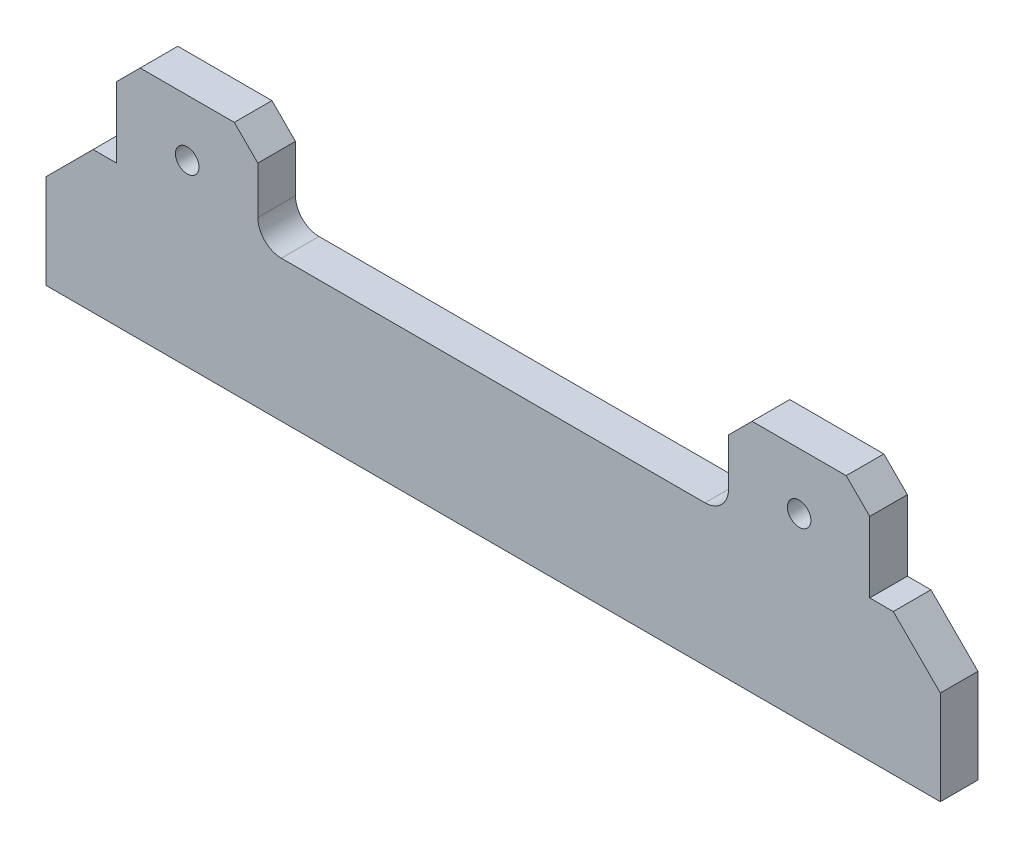
SolidWorks part; units mm, degrees
ref_plane "前视基准面" through (0, 0, 0) normal (0, 0, 1) x (1, 0, 0)
ref_plane "上视基准面" through (0, 0, 0) normal (0, 1, 0) x (1, 0, 0)
ref_plane "右视基准面" through (0, 0, 0) normal (1, 0, 0) x (0, 0, -1)
sketch "草图1" plane through (0, 0, 0) normal (0, 0, 1) x (1, 0, 0)
  line L1 (95, 25) -> (-95, 25)
  line L2 (95, 25) -> (95, -25)
  line L3 (95, -25) -> (-95, -25)
  line L4 (-95, 25) -> (-95, -25)
  line L5 (95, 25) -> (-95, -25) construction
  line L6 (95, -25) -> (-95, 25) construction
  point P0 (0, 0)
  dimension "D1" = 190
  dimension "D2" = 50
extrude "凸台-拉伸1" add sketch "草图1" along normal blind 8
sketch "草图2" plane through (0, 0, 8) normal (0, 0, 1) x (1, 0, 0)
  line L0 (-95, 25) -> (-95, -25) construction
  line L1 (-95, -5) -> (-85, 5)
  line L2 (-85, 5) -> (-80, 5)
  line L3 (-80, 5) -> (-80, 25)
  line L4 (95, 25) -> (-95, 25) construction
  line L5 (-80, 25) -> (-50, 25)
  line L6 (-50, 25) -> (-50, 5)
  line L7 (-50, 5) -> (50, 5)
  line L8 (50, 5) -> (50, 25)
  line L9 (50, 25) -> (80, 25)
  line L10 (80, 25) -> (80, 5)
  line L11 (80, 5) -> (85, 5)
  line L12 (85, 5) -> (95, -5)
  line L13 (95, -25) -> (95, 25) construction
  line L14 (-95, -5) -> (-95, 25)
  line L15 (-95, 25) -> (-3.8011, 36.2648)
  line L16 (-3.8011, 36.2648) -> (95, 25)
  line L17 (95, 25) -> (95, -5)
  dimension "D1" = 10
  dimension "D2" = 10
  dimension "D3" = 10
  dimension "D4" = 10
  dimension "D5" = 100
  dimension "D6" = 30
  dimension "D7" = 30
  dimension "D8" = 5
  dimension "D9" = 20
extrude "切除-拉伸1" cut sketch "草图2" against normal blind 8
chamfer "倒角1" distance 5 angle 45 4 edges at (80, 25, 4) (-50, 25, 4) (50, 25, 4) (-80, 25, 4)
sketch "草图3" plane through (0, 0, 8) normal (0, 0, 1) x (1, 0, 0)
  line L0 (-55, 25) -> (-75, 25) construction
  circle A0 centre (-65, 13) radius 2
  circle A1 centre (65, 13) radius 2
  dimension "D3" = 12
  dimension "D4" = 4
  dimension "D1" = 130
  dimension "D2" = 65
hole_wizard "M6 螺纹孔1" positions "草图4" profile "草图5" tap size "M6" standard "ISO" end condition through all
sketch "草图4" plane through (0, 0, 8) normal (0, 0, 1) x (1, 0, 0)
  point P0 (-65, 13)
  point P3 (65, 13)
sketch "草图5" plane through (-65, 13, 8) normal (1, 0, 0) x (0, -1, 0)
  line L0 (0, 0) -> (0, 8)
  line L1 (0, 8) -> (2.5, 8)
  line L2 (2.5, 8) -> (2.5, 0)
  line L5 (2.5, 0) -> (0, 0)
  line L11 (0, -6.35) -> (0, 107.95) construction
  dimension "通孔螺纹孔钻头直径" = 5
  dimension "通孔螺纹孔钻头深度" = 8
cosmetic thread "孔螺蚊线1" parameters "D2"=6
cosmetic thread "孔螺蚊线2" parameters "D2"=6
fillet "圆角1" radius 5 2 edges at (50, 5, 4) (-50, 5, 4)
